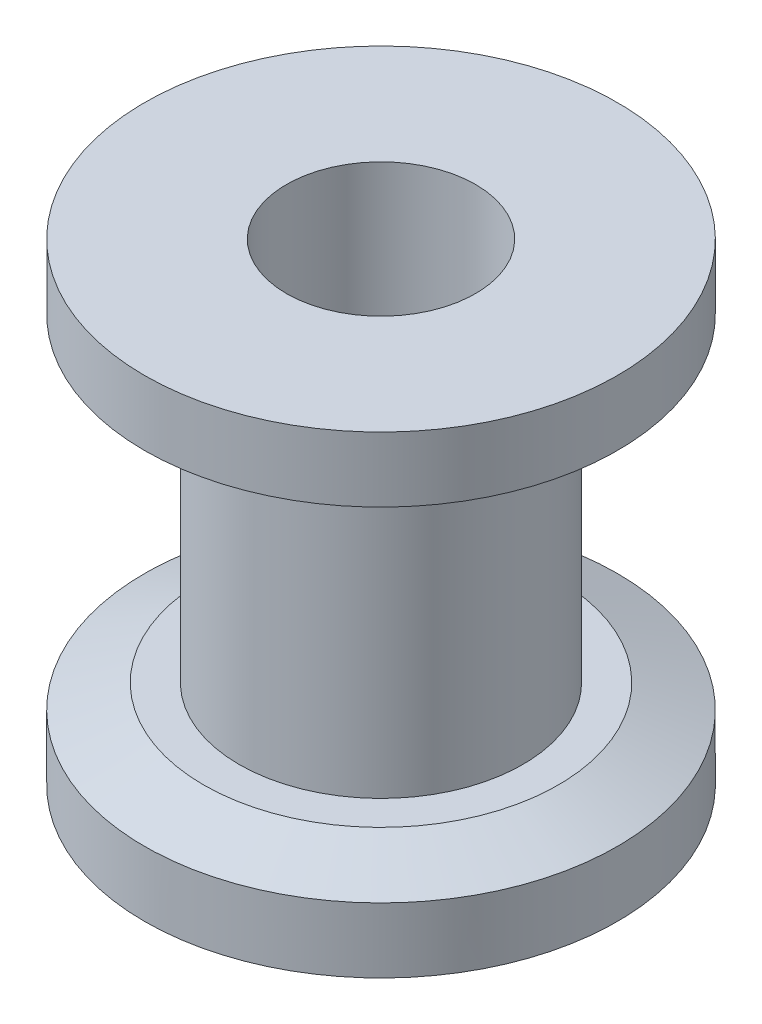
SolidWorks part; units mm, degrees
ref_plane "Front Plane" through (0, 0, 0) normal (0, 0, 1) x (1, 0, 0)
ref_plane "Top Plane" through (0, 0, 0) normal (0, 1, 0) x (1, 0, 0)
ref_plane "Right Plane" through (0, 0, 0) normal (1, 0, 0) x (0, 0, -1)
sketch "Sketch1" plane through (0, 0, 0) normal (0, 1, 0) x (1, 0, 0)
  circle A0 centre (0, 0) radius 20
  circle A1 centre (0, 0) radius 8
  dimension "D1" = 40
  dimension "D2" = 16
extrude "Boss-Extrude1" add sketch "Sketch1" along normal blind 40
sketch "Sketch2" plane through (0, 0, 0) normal (0, 0, 1) x (1, 0, 0)
  line L0 (0, 0) -> (0, 50000) construction
  line L1 (20, 0) -> (20, 40) construction
  line L2 (28, 7.5) -> (12, 7.5)
  line L3 (28, 7.5) -> (28, 32.5)
  line L4 (28, 32.5) -> (12, 32.5)
  line L5 (12, 7.5) -> (12, 32.5)
  line L6 (28, 7.5) -> (12, 32.5) construction
  line L7 (28, 32.5) -> (12, 7.5) construction
  point P3 (20, 20)
  dimension "D1" = 8
  dimension "D2" = 25
revolve "Cut-Revolve1" cut sketch "Sketch2" angle 360 about L0
chamfer "Chamfer1" distance 5 distance2 2 2 edges at (0, 32.5, 20) (0, 7.5, -20)
